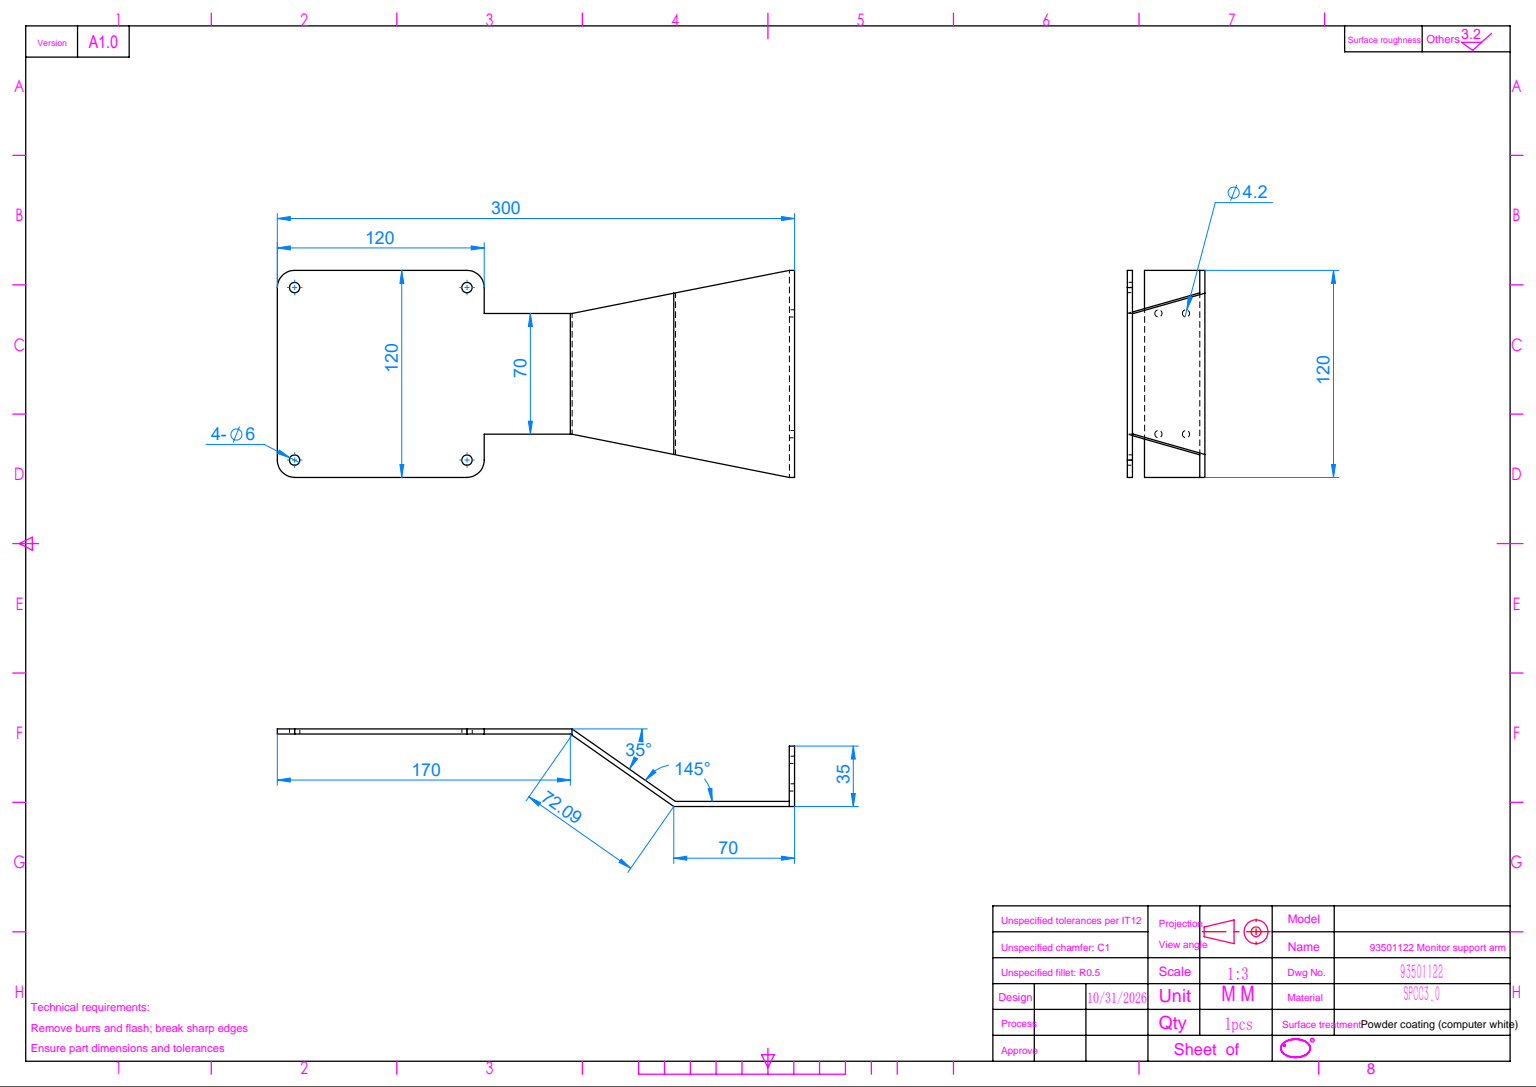
SolidWorks part; units mm, degrees
ref_plane "前视基准面" through (0, 0, 0) normal (0, 0, 1) x (1, 0, 0)
ref_plane "上视基准面" through (0, 0, 0) normal (0, 1, 0) x (1, 0, 0)
ref_plane "右视基准面" through (0, 0, 0) normal (1, 0, 0) x (0, 0, -1)
sketch "草图1" plane through (0, 0, 0) normal (0, 0, 1) x (1, 0, 0)
  line L0 (0, 0) -> (170, 0)
  line L1 (170, 0) -> (230, -42)
  line L2 (230, -42) -> (300, -42)
  line L3 (300, -42) -> (300, -7)
  dimension "D1" = 170
  dimension "D2" = 35
  dimension "D3" = 42
  dimension "D4" = 70
  dimension "D5" = 60
extrude "拉伸-薄壁1" add sketch "草图1" along normal blind 60 and the other way blind 60 thin thin type one direction reverse wall 3
sketch "草图2" plane through (0, 3, 0) normal (0, 1, 0) x (1, 0, 0)
  line L0 (120, 60) -> (120, 35)
  line L1 (0, 60) -> (170.9457, 60) construction
  line L2 (120, 35) -> (170.9457, 35)
  line L3 (170.9457, 60) -> (170.9457, -60) construction
  line L4 (170.9457, 35) -> (297, 60)
  line L5 (297, 60) -> (120, 60)
  line L6 (0, 0) -> (329.1432, 0) construction
  line L7 (297, -60) -> (120, -60)
  line L8 (170.9457, -35) -> (297, -60)
  line L9 (120, -35) -> (170.9457, -35)
  line L10 (120, -60) -> (120, -35)
  line L11 (0, 60) -> (0, -60) construction
  dimension "D1" = 120
  dimension "D2" = 70
extrude "切除-拉伸1" cut sketch "草图2" against normal through all
fillet "圆角1" radius 10 4 edges at (120, 1.5, 60) (0, 1.5, 60) (0, 1.5, -60) (120, 1.5, -60)
sketch "草图3" plane through (0, 3, 0) normal (0, 1, 0) x (1, 0, 0)
  circle A0 centre (10, 50) radius 3
  circle A1 centre (110, 50) radius 3
  circle A2 centre (110, -50) radius 3
  circle A3 centre (10, -50) radius 3
  dimension "D1" = 6
extrude "切除-拉伸2" cut sketch "草图3" against normal up to next
sketch "草图4" plane through (300, 0, 0) normal (1, 0, 0) x (0, 0, -1)
  line L0 (0, 0) -> (0, -42.4493) construction
  line L1 (60, -7) -> (-60, -7) construction
  circle A0 centre (-35, -15) radius 2.1
  circle A1 centre (-35, -31) radius 2.1
  circle A2 centre (35, -31) radius 2.1
  circle A3 centre (35, -15) radius 2.1
  dimension "D1" = 4.2
  dimension "D2" = 8
  dimension "D3" = 16
  dimension "D4" = 70
extrude "切除-拉伸3" cut sketch "草图4" against normal up to next
